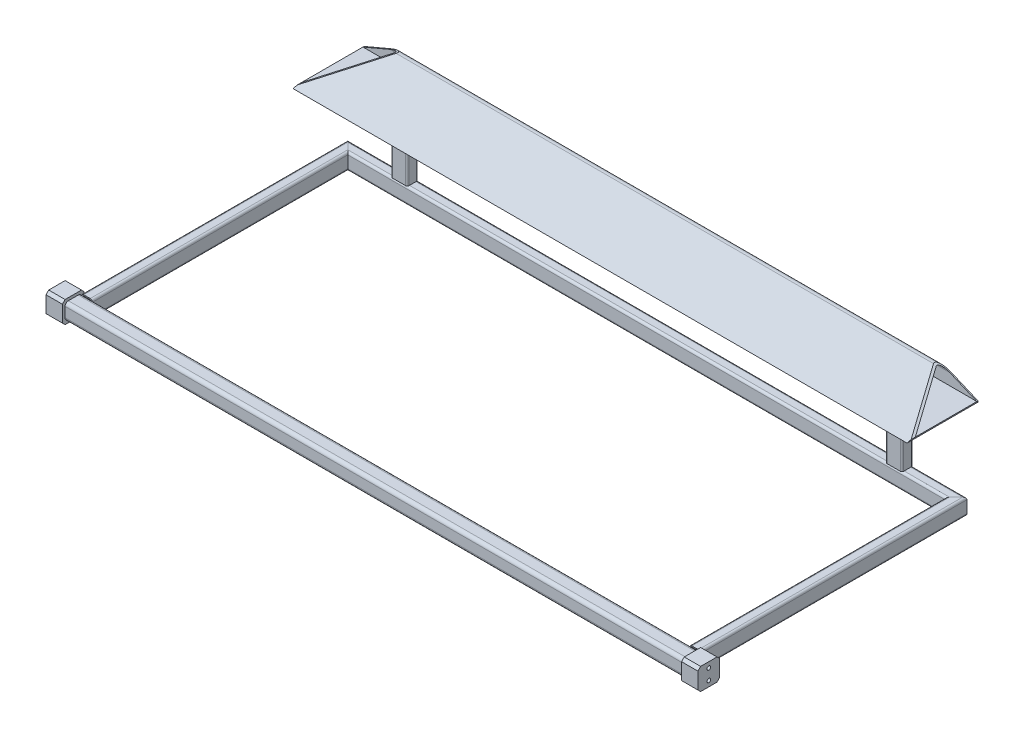
from build123d import *

# Parameters (mm, degrees)
COLD_FORMED_HOLLOW_SQUARE_STEEL_FOR_STRU_DEPTH = 1134.5
COLD_FORMED_HOLLOW_RECTANGULAR_STEEL_FOR_DEPTH = 497.034804644
COLD_FORMED_HOLLOW_RECTANGULAR_STEEL_3_DEPTH   = 1152.576663772
COLD_FORMED_HOLLOW_RECTANGULAR_STEEL_5_DEPTH   = 497.034804644
BOSS_EXTRUDE1_DEPTH                            = 30
SKETCH6_R                                      = 1
CUT_EXTRUDE1_DEPTH                             = 30
M8_TAPPED_HOLE1_AT_2_COUNT                     = 2
M8_TAPPED_HOLE1_AT_2_PITCH                     = 20
SKETCH_12_R                                    = 1
CUT_EXTRUDE4_DEPTH                             = 2
BOSS_EXTRUDE2_DEPTH                            = 162
BOSS_EXTRUDE2_2_DEPTH                          = 162
CUT_EXTRUDE6_DEPTH                             = 801.55169197
CUT_EXTRUDE6_DEPTH_BACK                        = 801.55169197
M6_TAPPED_HOLE1_AT_2_COUNT                     = 2
M6_TAPPED_HOLE1_AT_2_PITCH                     = 35
M6_TAPPED_HOLE1_AT_3_COUNT                     = 2
M6_TAPPED_HOLE1_AT_3_PITCH                     = 70
M6_TAPPED_HOLE1_AT_4_COUNT                     = 2
M6_TAPPED_HOLE1_AT_4_PITCH                     = 105
BOSS_EXTRUDE3_DEPTH                            = 562.5
CUT_EXTRUDE7_DEPTH                             = 373


with BuildPart() as part:
    # Sketch1 → Cold-formed hollow square steel for structures(gb t6728-2002) 30×3(1) (new body)
    with BuildSketch(Plane(origin=(0, 0, 0), x_dir=(0, 0, -1), z_dir=(1, 0, 0))):
        with BuildLine():
            Line((-9, -15), (9, -15))
            ThreePointArc((9, -15), (13.242640687, -13.242640687), (15, -9))
            Line((15, -9), (15, 9))
            ThreePointArc((15, 9), (13.242640687, 13.242640687), (9, 15))
            Line((9, 15), (-9, 15))
            ThreePointArc((-9, 15), (-13.242640687, 13.242640687), (-15, 9))
            Line((-15, 9), (-15, -9))
            ThreePointArc((-15, -9), (-13.242640687, -13.242640687), (-9, -15))
        make_face()
        with BuildLine():
            Line((-9, -12), (9, -12))
            ThreePointArc((9, -12), (11.121320344, -11.121320344), (12, -9))
            Line((12, -9), (12, 9))
            ThreePointArc((12, 9), (11.121320344, 11.121320344), (9, 12))
            Line((9, 12), (-9, 12))
            ThreePointArc((-9, 12), (-11.121320344, 11.121320344), (-12, 9))
            Line((-12, 9), (-12, -9))
            ThreePointArc((-12, -9), (-11.121320344, -11.121320344), (-9, -12))
        make_face(mode=Mode.SUBTRACT)
    extrude(amount=COLD_FORMED_HOLLOW_SQUARE_STEEL_FOR_STRU_DEPTH)


with BuildPart() as body_2:
    # Sketch12 → Cold-formed hollow rectangular steel for structures(gb t6728-2002) 30×20×2(2) (new body)
    with BuildSketch(Plane(origin=(9.989424491, -0.459780742, -14.992951733), x_dir=(1, 0, 0), z_dir=(0, 0, -1))):
        with BuildLine():
            Line((-6, -15), (6, -15))
            ThreePointArc((6, -15), (8.828427125, -13.828427125), (10, -11))
            Line((10, -11), (10, 11))
            ThreePointArc((10, 11), (8.828427125, 13.828427125), (6, 15))
            Line((6, 15), (-6, 15))
            ThreePointArc((-6, 15), (-8.828427125, 13.828427125), (-10, 11))
            Line((-10, 11), (-10, -11))
            ThreePointArc((-10, -11), (-8.828427125, -13.828427125), (-6, -15))
        make_face()
        with BuildLine():
            Line((-6, -13), (6, -13))
            ThreePointArc((6, -13), (7.414213562, -12.414213562), (8, -11))
            Line((8, -11), (8, 11))
            ThreePointArc((8, 11), (7.414213562, 12.414213562), (6, 13))
            Line((6, 13), (-6, 13))
            ThreePointArc((-6, 13), (-7.414213562, 12.414213562), (-8, 11))
            Line((-8, 11), (-8, -11))
            ThreePointArc((-8, -11), (-7.414213562, -12.414213562), (-6, -13))
        make_face(mode=Mode.SUBTRACT)
    extrude(amount=COLD_FORMED_HOLLOW_RECTANGULAR_STEEL_FOR_DEPTH)

    # Cold-formed hollow rectangular steel 2
    split(bisect_by=Plane(origin=(9.989424491, -0.459780742, -493), x_dir=(0, -1, 0), z_dir=(-0.707106781, 0, 0.707106781)), keep=Keep.TOP)


with BuildPart() as body_3:
    # Sketch12 on segment 2 (carried to segment 2) → Cold-formed hollow rectangular steel 3 (new body)
    with BuildSketch(Plane(origin=(-9.038331886, -0.459780742, -493), x_dir=(0, 0, 1), z_dir=(1, 0, 0))):
        with BuildLine():
            Line((-6, -15), (6, -15))
            ThreePointArc((6, -15), (8.828427125, -13.828427125), (10, -11))
            Line((10, -11), (10, 11))
            ThreePointArc((10, 11), (8.828427125, 13.828427125), (6, 15))
            Line((6, 15), (-6, 15))
            ThreePointArc((-6, 15), (-8.828427125, 13.828427125), (-10, 11))
            Line((-10, 11), (-10, -11))
            ThreePointArc((-10, -11), (-8.828427125, -13.828427125), (-6, -15))
        make_face()
        with BuildLine():
            Line((-6, -13), (6, -13))
            ThreePointArc((6, -13), (7.414213562, -12.414213562), (8, -11))
            Line((8, -11), (8, 11))
            ThreePointArc((8, 11), (7.414213562, 12.414213562), (6, 13))
            Line((6, 13), (-6, 13))
            ThreePointArc((-6, 13), (-7.414213562, 12.414213562), (-8, 11))
            Line((-8, 11), (-8, -11))
            ThreePointArc((-8, -11), (-7.414213562, -12.414213562), (-6, -13))
        make_face(mode=Mode.SUBTRACT)
    extrude(amount=COLD_FORMED_HOLLOW_RECTANGULAR_STEEL_3_DEPTH)

    # Cold-formed hollow rectangular steel 3 m
    split(bisect_by=Plane(origin=(9.989424491, -0.459780742, -493), x_dir=(0, 1, 0), z_dir=(0.707106781, 0, -0.707106781)), keep=Keep.TOP)

    # Cold-formed hollow rectangular steel 4
    split(bisect_by=Plane(origin=(1124.510575509, -0.459780742, -493), x_dir=(0, -1, 0), z_dir=(-0.707106781, 0, -0.707106781)), keep=Keep.TOP)

    # 草图12 → Cut-Extrude4 (cut)
    with BuildSketch(Plane.XY.offset(-503)):
        with Locations((689.510575509, 0)):
            Circle(SKETCH_12_R)
        with Locations((724.510575509, 0)):
            Circle(SKETCH_12_R)
        with Locations((759.510575509, 0)):
            Circle(SKETCH_12_R)
        with Locations((794.510575509, 0)):
            Circle(SKETCH_12_R)
    extrude(amount=CUT_EXTRUDE4_DEPTH, mode=Mode.SUBTRACT)

    # Sketch16 → M6 Tapped Hole1 (revolve, cut)
    with BuildSketch(Plane(origin=(794.510575509, 0, -503), x_dir=(0, 1, 0), z_dir=(1, 0, 0))):
        Polygon((0, 0), (0, 17), (2.5, 15.497848452), (2.5, 0), align=None)
    m6_tapped_hole1 = revolve(axis=Axis((794.510575509, 0, -509.35), (0, 0, 1)), mode=Mode.SUBTRACT)

    # M6 Tapped Hole1 at 2: M6 Tapped Hole1 ×2
    with Locations(*[(-i * M6_TAPPED_HOLE1_AT_2_PITCH, 0, 0) for i in range(1, M6_TAPPED_HOLE1_AT_2_COUNT)]):
        add(m6_tapped_hole1, mode=Mode.SUBTRACT)

    # M6 Tapped Hole1 at 3: M6 Tapped Hole1 ×2
    with Locations(*[(-i * M6_TAPPED_HOLE1_AT_3_PITCH, 0, 0) for i in range(1, M6_TAPPED_HOLE1_AT_3_COUNT)]):
        add(m6_tapped_hole1, mode=Mode.SUBTRACT)

    # M6 Tapped Hole1 at 4: M6 Tapped Hole1 ×2
    with Locations(*[(-i * M6_TAPPED_HOLE1_AT_4_PITCH, 0, 0) for i in range(1, M6_TAPPED_HOLE1_AT_4_COUNT)]):
        add(m6_tapped_hole1, mode=Mode.SUBTRACT)


with BuildPart() as body_4:
    # Sketch12 on segment 3 (carried to segment 3) → Cold-formed hollow rectangular steel 5 (new body)
    with BuildSketch(Plane(origin=(1124.510575509, -0.459780742, -512.027756377), x_dir=(-1, 0, 0), z_dir=(0, 0, 1))):
        with BuildLine():
            Line((-6, -15), (6, -15))
            ThreePointArc((6, -15), (8.828427125, -13.828427125), (10, -11))
            Line((10, -11), (10, 11))
            ThreePointArc((10, 11), (8.828427125, 13.828427125), (6, 15))
            Line((6, 15), (-6, 15))
            ThreePointArc((-6, 15), (-8.828427125, 13.828427125), (-10, 11))
            Line((-10, 11), (-10, -11))
            ThreePointArc((-10, -11), (-8.828427125, -13.828427125), (-6, -15))
        make_face()
        with BuildLine():
            Line((-6, -13), (6, -13))
            ThreePointArc((6, -13), (7.414213562, -12.414213562), (8, -11))
            Line((8, -11), (8, 11))
            ThreePointArc((8, 11), (7.414213562, 12.414213562), (6, 13))
            Line((6, 13), (-6, 13))
            ThreePointArc((-6, 13), (-7.414213562, 12.414213562), (-8, 11))
            Line((-8, 11), (-8, -11))
            ThreePointArc((-8, -11), (-7.414213562, -12.414213562), (-6, -13))
        make_face(mode=Mode.SUBTRACT)
    extrude(amount=COLD_FORMED_HOLLOW_RECTANGULAR_STEEL_5_DEPTH)

    # Cold-formed hollow rectangular steel 5 m
    split(bisect_by=Plane(origin=(1124.510575509, -0.459780742, -493), x_dir=(0, 1, 0), z_dir=(0.707106781, 0, 0.707106781)), keep=Keep.TOP)


with BuildPart() as body_5:
    # Sketch5 → Boss-Extrude1 (new body)
    with BuildSketch(Plane.ZY):
        Polygon((-20, 15), (-15, 20), (15, 20), (20, 15), (20, -15), (15, -20), (-15, -20), (-20, -15), align=None)
    boss_extrude1 = extrude(amount=BOSS_EXTRUDE1_DEPTH)

    # Sketch6 → Cut-Extrude1 (cut)
    with BuildSketch(Plane.ZY.offset(30)):
        with Locations((0, 10)):
            Circle(SKETCH6_R)
        with Locations((0, -10)):
            Circle(SKETCH6_R)
    cut_extrude1 = extrude(amount=-CUT_EXTRUDE1_DEPTH, mode=Mode.SUBTRACT)


with BuildPart() as m8_tapped_hole1_tool:
    # Sketch7 → M8 Tapped Hole1 (revolve)
    with BuildSketch(Plane(origin=(-30, 10, 0), x_dir=(0, 0, 1), z_dir=(0, 1, 0))):
        Polygon((0, 0), (0, 32.042926105), (3.4, 30), (3.4, 0), align=None)
    m8_tapped_hole1 = revolve(axis=Axis((-36.35, 10, 0), (1, 0, 0)))


with BuildPart() as part_1:
    add(part.part)

    # M8 Tapped Hole1: cut by m8_tapped_hole1_tool
    add(m8_tapped_hole1_tool.part, mode=Mode.SUBTRACT)


with BuildPart() as body_5_1:
    add(body_5.part)

    # M8 Tapped Hole1: cut by m8_tapped_hole1_tool
    add(m8_tapped_hole1_tool.part, mode=Mode.SUBTRACT)


with BuildPart() as m8_tapped_hole1_at_2_tool:
    # M8 Tapped Hole1 at 2: M8 Tapped Hole1 ×2
    with Locations(*[(0, -i * M8_TAPPED_HOLE1_AT_2_PITCH, 0) for i in range(1, M8_TAPPED_HOLE1_AT_2_COUNT)]):
        add(m8_tapped_hole1)


with BuildPart() as part_2:
    add(part_1.part)

    # M8 Tapped Hole1 at 2: cut by m8_tapped_hole1_at_2_tool
    add(m8_tapped_hole1_at_2_tool.part, mode=Mode.SUBTRACT)


    add(body_4.part)  # Mirror1 merges body 4
    # Mirror1: Boss-Extrude1, Cut-Extrude1, M8 Tapped Hole1 across plane
    add(boss_extrude1.mirror(Plane.ZY.offset(-567.25)))
    add(cut_extrude1.mirror(Plane.ZY.offset(-567.25)), mode=Mode.SUBTRACT)
    add(m8_tapped_hole1.mirror(Plane.ZY.offset(-567.25)), mode=Mode.SUBTRACT)

    # Mirror1 copy 1 sketch → Mirror1 copy 1 (revolve, cut)
    with BuildSketch(Plane(origin=(1164.5, -10, 0), x_dir=(0, 0, 1), z_dir=(0, 1, 0))):
        Polygon((0, 0), (0, -32.042926105), (3.4, -30), (3.4, 0), align=None)
    revolve(axis=Axis((1170.85, -10, 0), (1, 0, 0)), mode=Mode.SUBTRACT)


with BuildPart() as body_5_2:
    add(body_5_1.part)

    # M8 Tapped Hole1 at 2: cut by m8_tapped_hole1_at_2_tool
    add(m8_tapped_hole1_at_2_tool.part, mode=Mode.SUBTRACT)


with BuildPart() as body_5_2_1:
    # Sketch14 → Boss-Extrude2 (new body)
    with BuildSketch(Plane(origin=(0, 14.540219258, 0), x_dir=(1, 0, 0), z_dir=(0, 1, 0))):
        with BuildLine():
            Line((1008.5, 503), (1032.5, 503))
            ThreePointArc((1032.5, 503), (1034.621320344, 502.121320344), (1035.5, 500))
            Line((1035.5, 500), (1035.5, 486))
            ThreePointArc((1035.5, 486), (1034.621320344, 483.878679656), (1032.5, 483))
            Line((1032.5, 483), (1008.5, 483))
            ThreePointArc((1008.5, 483), (1006.378679656, 483.878679656), (1005.5, 486))
            Line((1005.5, 486), (1005.5, 500))
            ThreePointArc((1005.5, 500), (1006.378679656, 502.121320344), (1008.5, 503))
        make_face()
        with BuildLine():
            Line((1033.5, 500), (1033.5, 486))
            ThreePointArc((1033.5, 486), (1033.207106781, 485.292893219), (1032.5, 485))
            Line((1032.5, 485), (1008.5, 485))
            ThreePointArc((1008.5, 485), (1007.792893219, 485.292893219), (1007.5, 486))
            Line((1007.5, 486), (1007.5, 500))
            ThreePointArc((1007.5, 500), (1007.792893219, 500.707106781), (1008.5, 501))
            Line((1008.5, 501), (1032.5, 501))
            ThreePointArc((1032.5, 501), (1033.207106781, 500.707106781), (1033.5, 500))
        make_face(mode=Mode.SUBTRACT)
    extrude(amount=BOSS_EXTRUDE2_DEPTH)


with BuildPart() as body_6:
    # Sketch14 → Boss-Extrude2 2 (new body)
    with BuildSketch(Plane(origin=(0, 14.540219258, 0), x_dir=(1, 0, 0), z_dir=(0, 1, 0))):
        with BuildLine():
            Line((99, 500), (99, 486))
            ThreePointArc((99, 486), (99.878679656, 483.878679656), (102, 483))
            Line((102, 483), (126, 483))
            ThreePointArc((126, 483), (128.121320344, 483.878679656), (129, 486))
            Line((129, 486), (129, 500))
            ThreePointArc((129, 500), (128.121320344, 502.121320344), (126, 503))
            Line((126, 503), (102, 503))
            ThreePointArc((102, 503), (99.878679656, 502.121320344), (99, 500))
        make_face()
        with BuildLine():
            Line((126, 485), (102, 485))
            ThreePointArc((102, 485), (101.292893219, 485.292893219), (101, 486))
            Line((101, 486), (101, 500))
            ThreePointArc((101, 500), (101.292893219, 500.707106781), (102, 501))
            Line((102, 501), (126, 501))
            ThreePointArc((126, 501), (126.707106781, 500.707106781), (127, 500))
            Line((127, 500), (127, 486))
            ThreePointArc((127, 486), (126.707106781, 485.292893219), (126, 485))
        make_face(mode=Mode.SUBTRACT)
    extrude(amount=BOSS_EXTRUDE2_2_DEPTH)


with BuildPart() as cut_extrude6_tool:
    # Sketch15 → Cut-Extrude6 (new, two sides: drawn at the far end of the back side and taken through both)
    with BuildSketch(Plane.ZY.offset(-567.25).offset(-CUT_EXTRUDE6_DEPTH_BACK)):
        Polygon((-503, 176.540219258), (-483, 176.540219258), (-483, 171.18123541), align=None)
    extrude(amount=CUT_EXTRUDE6_DEPTH + CUT_EXTRUDE6_DEPTH_BACK)


with BuildPart() as body_5_2_2:
    add(body_5_2_1.part)

    # Cut-Extrude6: cut by cut_extrude6_tool
    add(cut_extrude6_tool.part, mode=Mode.SUBTRACT)


with BuildPart() as body_6_1:
    add(body_6.part)

    # Cut-Extrude6: cut by cut_extrude6_tool
    add(cut_extrude6_tool.part, mode=Mode.SUBTRACT)


with BuildPart() as body_7:
    # Sketch17 → Boss-Extrude3 (new, symmetric)
    with BuildSketch(Plane.ZY.offset(-567.25)):
        with BuildLine():
            Line((-398, 150.476106414), (-516.569818141, 182.246793432))
            ThreePointArc((-516.569818141, 182.246793432), (-524.447521164, 180.679820874), (-528, 173.476106414))
            Line((-528, 173.476106414), (-528, 150.476106414))
            Line((-528, 150.476106414), (-398, 150.476106414))
        make_face()
        with BuildLine():
            Line((-413.191508225, 152.476106414), (-517.087456232, 180.314941779))
            ThreePointArc((-517.087456232, 180.314941779), (-523.229998306, 179.093114193), (-526, 173.476106414))
            Line((-526, 173.476106414), (-526, 152.476106414))
            Line((-526, 152.476106414), (-413.191508225, 152.476106414))
        make_face(mode=Mode.SUBTRACT)
    extrude(amount=BOSS_EXTRUDE3_DEPTH, both=True)

    # Sketch20 → Cut-Extrude7 (cut)
    with BuildSketch(Plane(origin=(0, 0, -528), x_dir=(-1, 0, 0), z_dir=(0, 0, -1))):
        Polygon((-1129.75, 152.476106414), (-1044.75, 188.556465792), (-1129.75, 188.556465792), align=None)
        Polygon((-89.75, 188.556465792), (-4.75, 188.556465792), (-4.75, 152.476106414), align=None)
    extrude(amount=-CUT_EXTRUDE7_DEPTH, mode=Mode.SUBTRACT)


solid = Compound([body_2.part, body_3.part, part_2.part, body_5_2.part, body_5_2_2.part, body_6_1.part, body_7.part])
